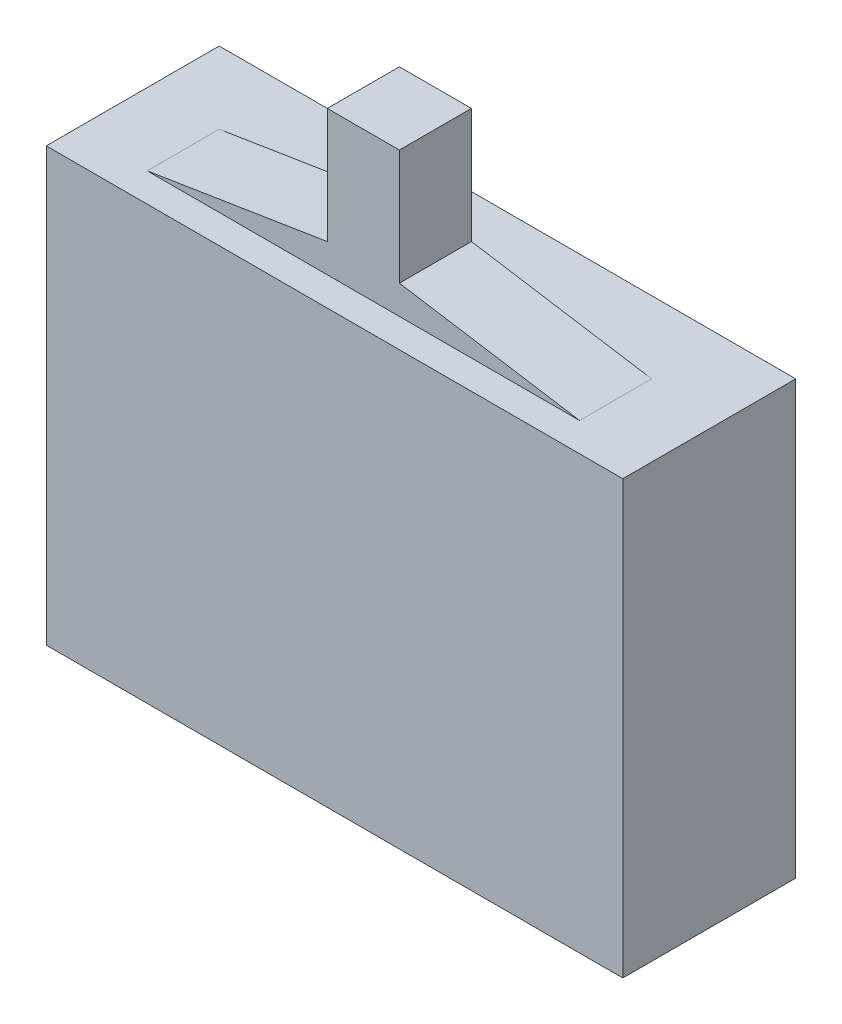
SolidWorks part; units mm, degrees
ref_plane "Front Plane" through (0, 0, 0) normal (0, 0, 1) x (1, 0, 0)
ref_plane "Top Plane" through (0, 0, 0) normal (0, 1, 0) x (1, 0, 0)
ref_plane "Right Plane" through (0, 0, 0) normal (1, 0, 0) x (0, 0, -1)
sketch "Sketch1" plane through (0, 0, 0) normal (0, 0, 1) x (1, 0, 0)
  line L1 (0, 0) -> (40, 0)
  line L2 (0, 0) -> (0, -30)
  line L3 (0, -30) -> (40, -30)
  line L4 (40, 0) -> (40, -30)
  line L5 (0, 0) -> (40, -30) construction
  line L6 (0, -30) -> (40, 0) construction
  point P4 (20, -15)
  dimension "D1" = 30
  dimension "D2" = 40
extrude "Boss-Extrude1" add sketch "Sketch1" along normal blind 12
sketch "Sketch2" plane through (0, 0, 0) normal (0, 0, 1) x (1, 0, 0)
  line L0 (22.5, 2) -> (22.5, 10)
  line L5 (20, 2) -> (20, 0) construction
  line L6 (5, 0) -> (35, 0)
  line L8 (17.5, 2) -> (22.5, 2)
  line L10 (5, 0) -> (22.5, 2) construction
  line L11 (17.5, 2) -> (35, 0) construction
  line L12 (17.5, 2) -> (5, 0)
  line L13 (22.5, 2) -> (35, 0)
  line L14 (22.5, 10) -> (17.5, 10)
  line L15 (17.5, 10) -> (17.5, 2)
  point P4 (20, 1.7143)
  dimension "D2" = 8
  dimension "5" = 5
  dimension "D3" = 2
  dimension "D4" = 30
  dimension "D5" = 5
extrude "Boss-Extrude3" add sketch "Sketch2" along normal blind 5 from offset 5
